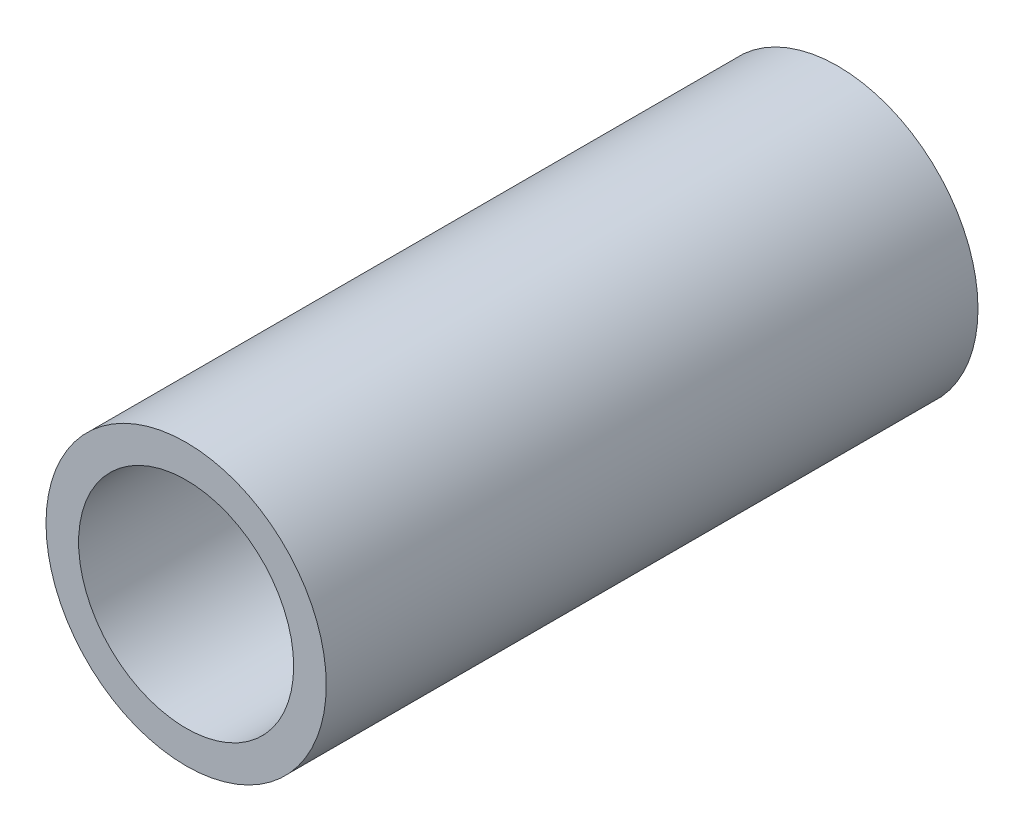
SolidWorks part; units mm, degrees
ref_plane "前视基准面" through (0, 0, 0) normal (0, 0, 1) x (1, 0, 0)
ref_plane "上视基准面" through (0, 0, 0) normal (0, 1, 0) x (1, 0, 0)
ref_plane "右视基准面" through (0, 0, 0) normal (1, 0, 0) x (0, 0, -1)
sketch "草图1" plane through (0, 0, 0) normal (0, 0, 1) x (1, 0, 0)
  circle A0 centre (0, 0) radius 21.5
  circle A1 centre (0, 0) radius 16.5
  dimension "D1" = 33
  dimension "D2" = 5
extrude "凸台-拉伸1" add sketch "草图1" along normal blind 100
